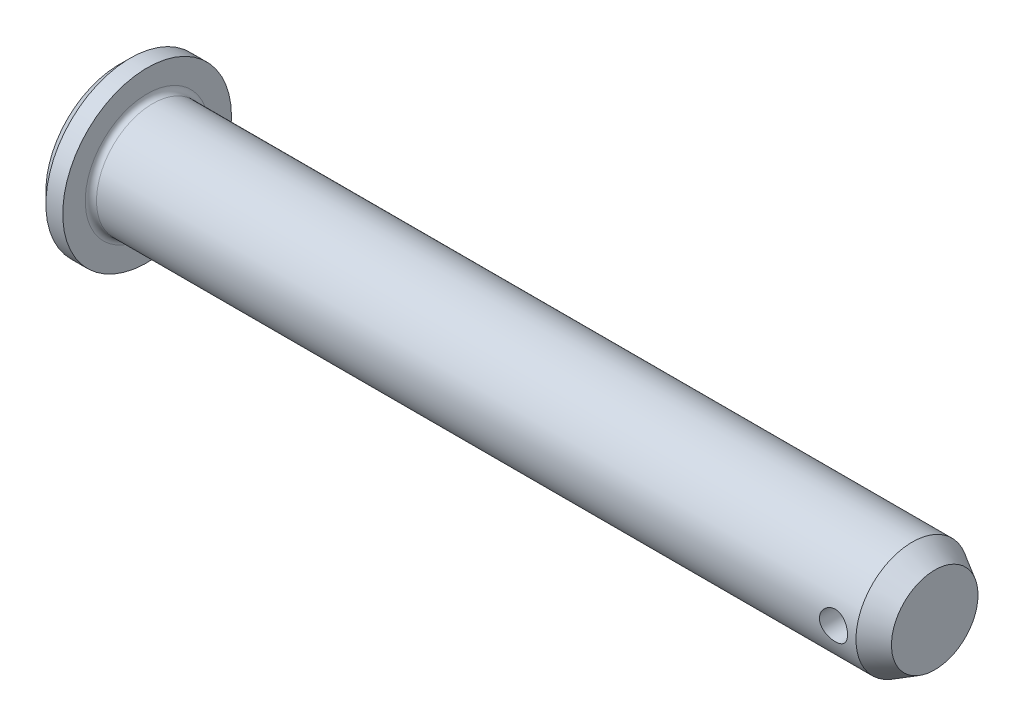
SolidWorks part; units mm, degrees
ref_plane "Front" through (0, 0, 0) normal (0, 0, 1) x (1, 0, 0)
ref_plane "Top" through (0, 0, 0) normal (0, 1, 0) x (1, 0, 0)
ref_plane "Right" through (0, 0, 0) normal (1, 0, 0) x (0, 0, -1)
sketch "Dimension sketch" plane through (0, 0, 0) normal (0, 0, 1) x (1, 0, 0)
  line L0 (0, 30) -> (0, 0)
  line L1 (0, 0) -> (140, 0)
  circle A0 centre (132, 0) radius 2.5 construction
  point P3 (0, 20)
  point P5 (5, 0)
  point P6 (1, 0)
  point P7 (136, 0)
  point P8 (7, 0)
  dimension "d1" = 5
  dimension "l" = 140
  dimension "dk" = 30
  dimension "d" = 20
  dimension "k" = 5
  dimension "r" = 1
  dimension "c" = 4
  dimension "e" = 2
  dimension "le" = 8
sketch "Sketch1" plane through (0, 0, 0) normal (0, 0, 1) x (1, 0, 0)
  line L0 (0, 0) -> (-7.3443, 0) construction
  line L1 (0, 0) -> (145, 0)
  line L2 (0, 0) -> (0, 13)
  line L3 (2, 15) -> (5, 15)
  line L4 (5, 15) -> (5, 10)
  line L5 (5, 10) -> (145, 10)
  line L6 (145, 10) -> (145, 0)
  line L7 (0, 13) -> (2, 15)
  point P4 (0, 15)
  dimension "D2" = 30
  dimension "D1" = 140
  dimension "D3" = 20
  dimension "D4" = 5
revolve "Base-Revolve" add sketch "Sketch1" angle 360 about L0
sketch "Sketch2" plane through (0, 0, 0) normal (0, 0, 1) x (1, 0, 0)
  line L0 (0, 0) -> (140, 0) construction
  line L1 (145, -10) -> (145, 10) construction
  circle A1 centre (137, 0) radius 2.5
  dimension "D1" = 5
  dimension "D2" = 8
extrude "Cut-Extrude1" cut sketch "Sketch2" against normal through all and the other way through all
fillet "Fillet1" radius 1 1 edges at (5, 0, -10)
chamfer "Chamfer1" distance 4 angle 30 1 edges at (145, 0, -10)
